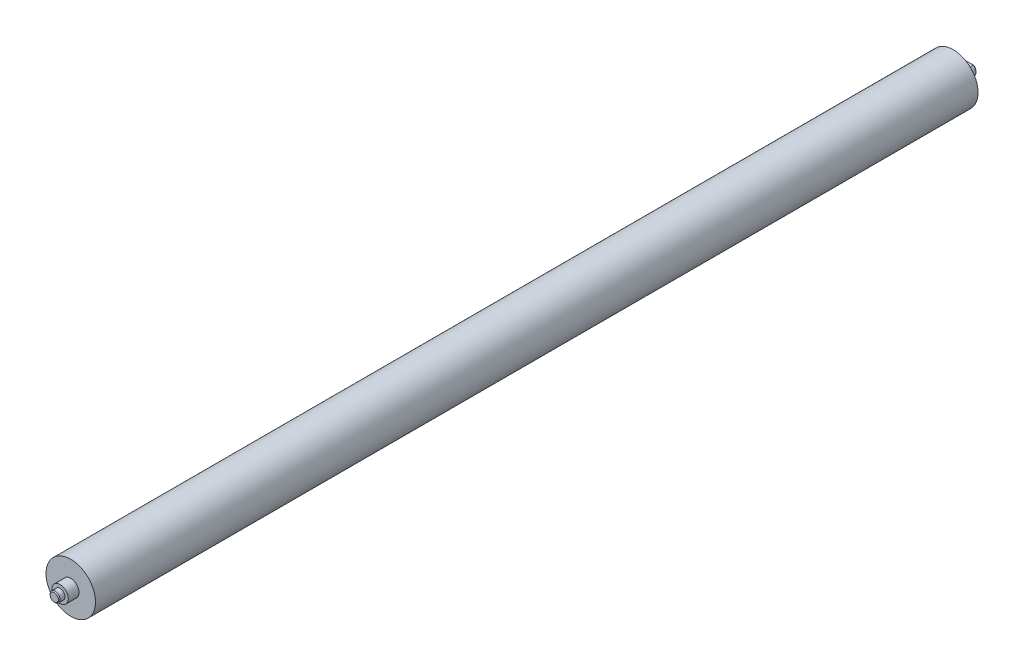
SolidWorks part; units mm, degrees
material "1023 碳钢板 (SS)"
ref_plane "Front Plane" through (0, 0, 0) normal (0, 0, 1) x (1, 0, 0)
ref_plane "Top Plane" through (0, 0, 0) normal (0, 1, 0) x (1, 0, 0)
ref_plane "Right Plane" through (0, 0, 0) normal (1, 0, 0) x (0, 0, -1)
ref_plane "Plane4" through (0, 0, 0) normal (0, -1, 0) x (1, 0, 0)
sketch "Sketch1" plane through (0, 0, 0) normal (0, -1, 0) x (1, 0, 0)
  line L0 (30, 535) -> (0, 535)
  line L1 (0, 535) -> (0, -535)
  line L2 (0, -535) -> (30, -535)
  line L3 (30, -535) -> (30, 535)
  line L4 (0, 535) -> (0, -535) construction
revolve "Revolve1" add sketch "Sketch1" angle 360 about L4
sketch "Sketch2" plane through (0, 0, -535) normal (0, 0, -1) x (-1, 0, 0)
  circle A0 centre (0, 0) radius 10
extrude "Boss-Extrude1" add sketch "Sketch2" along normal blind 6
sketch "Sketch3" plane through (0, 0, -541) normal (0, 0, -1) x (-1, 0, 0)
  line L0 (-4.5, 6) -> (4.5, 6)
  line L1 (4.5, -6) -> (-4.5, -6)
  arc A0 (-4.5, -6) -> (-4.5, 6) centre (0, 0) cw
  arc A1 (4.5, 6) -> (4.5, -6) centre (0, 0) cw
extrude "Boss-Extrude2" add sketch "Sketch3" along normal blind 15
sketch "Sketch4" plane through (0, 0, 535) normal (0, 0, 1) x (1, 0, 0)
  circle A0 centre (0, 0) radius 10
extrude "Boss-Extrude3" add sketch "Sketch4" along normal blind 13
sketch "Sketch5" plane through (0, 0, 548) normal (0, 0, 1) x (1, 0, 0)
  circle A0 centre (0, 0) radius 6
extrude "Boss-Extrude4" add sketch "Sketch5" along normal blind 7
chamfer "Chamfer1" distance 1 angle 45 5 edges at (0, 6, -556) (7.5, 0, -556) (-7.5, 0, -556) (0, -6, -556) (6, 0, 555)
